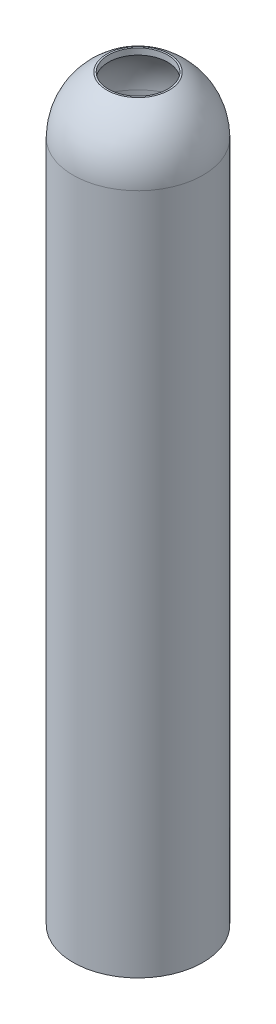
from build123d import *


with BuildPart() as part:
    # Sketch1 → Revolve1 (revolve)
    with BuildSketch(Plane.XY, mode=Mode.PRIVATE) as revolve1_sk:
        with BuildLine():
            Line((-2.18, 0), (-2.18, 22.889528854))
            ThreePointArc((-2.18, 22.889528854), (-1.876352845, 23.999348659), (-1.05, 24.8))
            Line((-1.05, 24.8), (-0.994634547, 24.8))
            Line((-0.994634547, 24.8), (-0.994634547, 24.59))
            ThreePointArc((-0.994634547, 24.59), (-1.708849036, 23.869699743), (-1.97, 22.889528854))
            Line((-1.97, 22.889528854), (-1.97, 0))
            Line((-1.97, 0), (-2.18, 0))
        make_face()
    revolve(revolve1_sk.sketch.rotate(Axis((0, 0, 0), (0, 1, 0)), 270), axis=Axis((0, 0, 0), (0, 1, 0)))


solid = part.part
